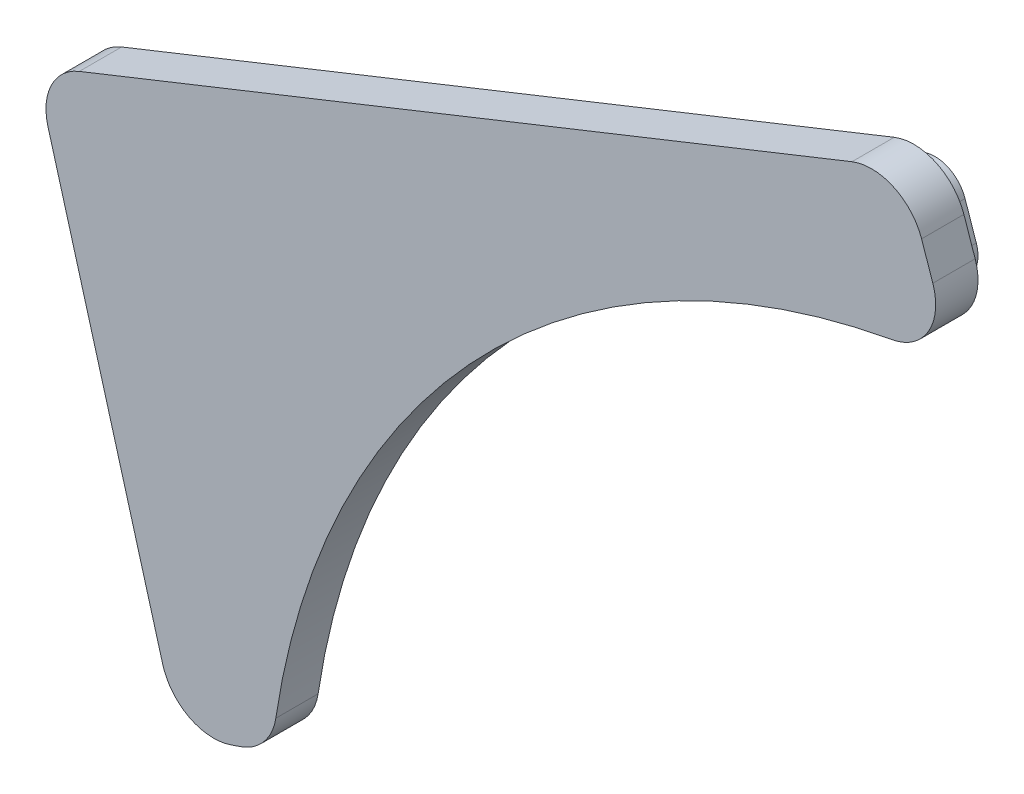
from build123d import *

# Parameters (mm, degrees)
EXTRUDE_1_DEPTH = 2
EXTRUDE_2_DEPTH = 4


with BuildPart() as part:
    # 草图1 → 凸台-拉伸1 (new body)
    with BuildSketch(Plane.XY):
        with BuildLine():
            Line((137.488957816, 148.560574876), (148.33581351, 109.973924886))
            ThreePointArc((148.33581351, 109.973924886), (149.830188599, 108.129149559), (152.197376559, 107.948113442))
            Line((152.197376559, 107.948113442), (153.12452466, 108.266185323))
            ThreePointArc((153.12452466, 108.266185323), (154.455434588, 109.182984766), (155.117593814, 110.657226135))
            ThreePointArc((155.117593814, 110.657226135), (175.157111586, 151.143900213), (214.998888251, 172.436760111))
            ThreePointArc((214.998888251, 172.436760111), (217.048600661, 173.871762608), (217.297595906, 176.361452247))
            Line((217.297595906, 176.361452247), (216.233642795, 179.462770427))
            ThreePointArc((216.233642795, 179.462770427), (214.647795853, 181.215617846), (212.284799547, 181.275892717))
            Line((212.284799547, 181.275892717), (139.265834382, 152.159042969))
            ThreePointArc((139.265834382, 152.159042969), (137.68708728, 150.700674405), (137.488957816, 148.560574876))
        make_face()
    extrude(amount=-EXTRUDE_1_DEPTH)

    # 草图2 → 凸台-拉伸2 (add)
    with BuildSketch(Plane.XY):
        with BuildLine():
            Line((153.773524821, 106.374413986), (152.84637672, 106.056342105))
            ThreePointArc((152.84637672, 106.056342105), (148.901063453, 106.358068967), (146.410438304, 109.432694512))
            Line((146.410438304, 109.432694512), (135.563582611, 148.019344502))
            ThreePointArc((135.563582611, 148.019344502), (135.893798384, 151.586177051), (138.525043553, 154.016791324))
            Line((138.525043553, 154.016791324), (211.544008718, 183.133641072))
            ThreePointArc((211.544008718, 183.133641072), (215.482335894, 183.033182953), (218.125414132, 180.111770588))
            Line((218.125414132, 180.111770588), (219.189367243, 177.010452408))
            ThreePointArc((219.189367243, 177.010452408), (218.774375168, 172.860969677), (215.358187818, 170.469298848))
            ThreePointArc((215.358187818, 170.469298848), (176.593215928, 149.75192165), (157.095306744, 110.359482007))
            ThreePointArc((157.095306744, 110.359482007), (155.991708034, 107.902413058), (153.773524821, 106.374413986))
        make_face()
    extrude(amount=EXTRUDE_2_DEPTH)


solid = part.part
